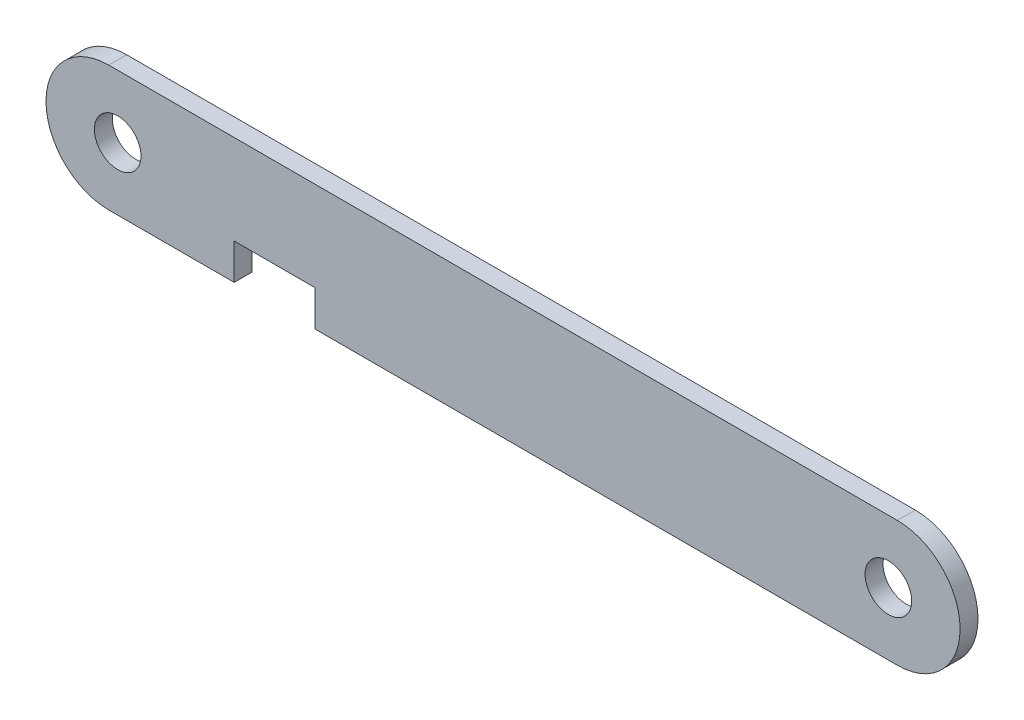
from build123d import *

# Parameters (mm, degrees)
SKETCH1_R      = 2.6
EXTRUDE1_DEPTH = 2


with BuildPart() as part:
    # Sketch1 → Extrude1 (new body)
    with BuildSketch(Plane.XY):
        with BuildLine():
            Line((-30, -7), (-30, -3))
            Line((-30, -3), (-21, -3))
            Line((-21, -3), (-21, -7))
            Line((-21, -7), (44, -7))
            ThreePointArc((44, -7), (51, 0), (44, 7))
            Line((44, 7), (-44, 7))
            ThreePointArc((-44, 7), (-51, 0), (-44, -7))
            Line((-44, -7), (-30, -7))
        make_face()
        with Locations(Location((-43, 0, 0), (0, 0, 180))):
            Circle(SKETCH1_R, mode=Mode.SUBTRACT)
        with Locations(Location((43, 0, 0), (0, 0, 180))):
            Circle(SKETCH1_R, mode=Mode.SUBTRACT)
    extrude(amount=EXTRUDE1_DEPTH)


solid = part.part
